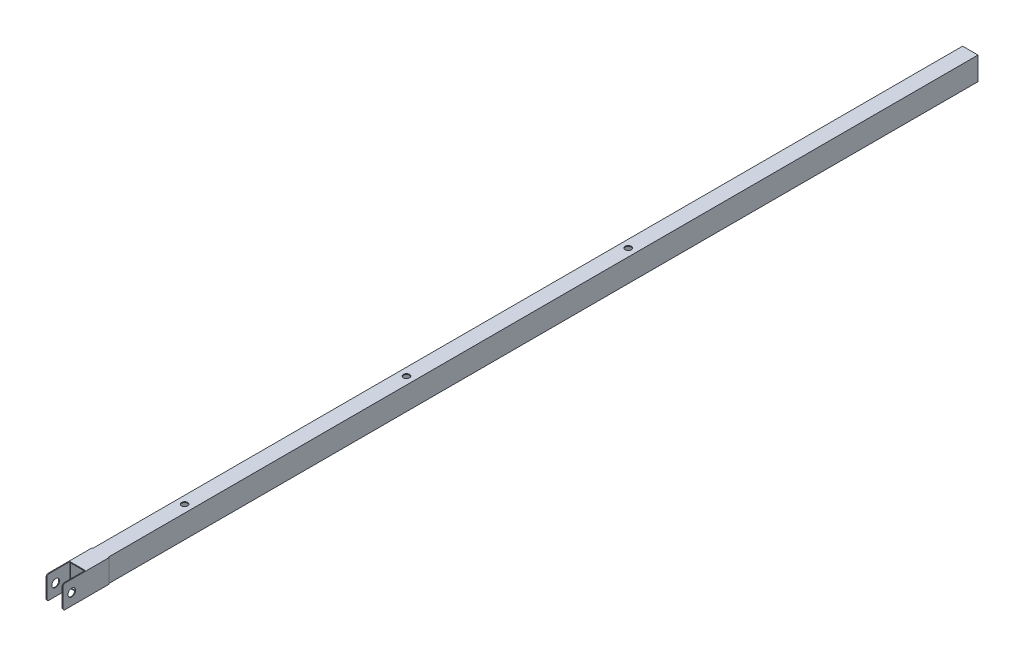
SolidWorks part; units mm, degrees
ref_plane "Front Plane" through (0, 0, 0) normal (0, 0, 1) x (1, 0, 0)
ref_plane "Top Plane" through (0, 0, 0) normal (0, 1, 0) x (1, 0, 0)
ref_plane "Right Plane" through (0, 0, 0) normal (1, 0, 0) x (0, 0, -1)
sketch "Sketch1" plane through (0, 0, 0) normal (0, 0, 1) x (1, 0, 0)
  line L1 (0, 0) -> (20, 0)
  line L2 (0, 0) -> (0, -30)
  line L3 (0, -30) -> (20, -30)
  line L4 (20, 0) -> (20, -30)
  line L8 (1, -1) -> (19, -1)
  line L9 (19, -1) -> (19, -29)
  line L10 (1, -29) -> (19, -29)
  line L11 (1, -1) -> (1, -29)
  dimension "D1" = 20
  dimension "D2" = 30
  dimension "D3" = 1
extrude "Boss-Extrude1" add sketch "Sketch1" along normal blind 859
sketch "Sketch3" plane through (0, 0, 0) normal (-1, 0, 0) x (0, 0, 1)
  line L0 (829, -30) -> (859, -30)
  line L2 (889, -27) -> (889, -3)
  line L3 (886, 0) -> (859, 0)
  line L4 (859, 0) -> (829, 0)
  line L5 (859, 0) -> (0, 0) construction
  line L6 (859, -30) -> (0, -30) construction
  line L7 (859, -30) -> (886, -30)
  line L8 (829, -30) -> (829, 0)
  arc A0 (889, -27) -> (886, -30) centre (886, -27) cw
  arc A1 (889, -3) -> (886, 0) centre (886, -3) ccw
  point P14 (889, -30)
  dimension "D3" = 3
  dimension "D4" = 3
  dimension "D1" = 30
  dimension "D2" = 30
extrude "Boss-Extrude2" add sketch "Sketch3" along normal blind 1
ref_plane "Plane4" through (10, 0, 0) normal (1, 0, 0) x (0, 0, -1)
mirror "Mirror2" about plane through (10, 0, 0) normal (1, 0, 0) of "Boss-Extrude2"
sketch "Sketch4" plane through (21, 0, 0) normal (1, 0, 0) x (0, 0, -1)
  line L0 (-889, -15) -> (-829, -15) construction
  line L1 (-889, -27) -> (-889, -3) construction
  line L2 (-829, 0) -> (-829, -30) construction
  line L3 (-857.5, 0) -> (-857.5, -30) construction
  line L4 (-886, 0) -> (-829, 0) construction
  line L5 (-829, -30) -> (-886, -30) construction
  circle A0 centre (-877.5, -15) radius 5
  dimension "D2" = 10
  dimension "D1" = 20
extrude "Cut-Extrude1" cut sketch "Sketch4" against normal through all
sketch "Sketch5" plane through (0, 0, 0) normal (0, 1, 0) x (1, 0, 0)
  line L0 (10, 0) -> (10, -859) construction
  line L2 (20, 0) -> (0, 0) construction
  line L3 (20, -859) -> (0, -859) construction
  circle A0 centre (10, -144) radius 4
  circle A1 centre (10, -432) radius 4
  circle A2 centre (10, -720) radius 4
  dimension "D1" = 8
  dimension "D3" = 8
  dimension "D5" = 8
  dimension "D2" = 144
  dimension "D4" = 288
  dimension "D6" = 288
extrude "Cut-Extrude2" cut sketch "Sketch5" against normal through all
sketch "Sketch6" plane through (0, 0, 0) normal (0, 0, -1) x (-1, 0, 0)
  line L0 (-1, -29) -> (-19, -29) construction
  line L1 (-1, -29) -> (-19, -29)
  line L2 (-19, -1) -> (-1, -1) construction
  line L3 (-19, -29) -> (-19, -1) construction
  line L4 (0, -30) -> (0, 0)
  line L5 (0, 0) -> (-20, 0)
  line L6 (-20, 0) -> (-20, -30)
  line L7 (-20, -30) -> (0, -30)
  line L8 (0, -30) -> (0, 0)
  line L9 (0, 0) -> (-20, 0)
  line L10 (-20, 0) -> (-20, -30)
  line L11 (-20, -30) -> (0, -30)
  line L12 (-1, -1) -> (-1, -29) construction
  line L13 (-19, -1) -> (-1, -1)
  line L14 (-19, -29) -> (-19, -1)
  line L15 (-1, -1) -> (-1, -29)
  dimension "D1" = 0
extrude "Boss-Extrude3" add sketch "Sketch6" along normal blind 300
